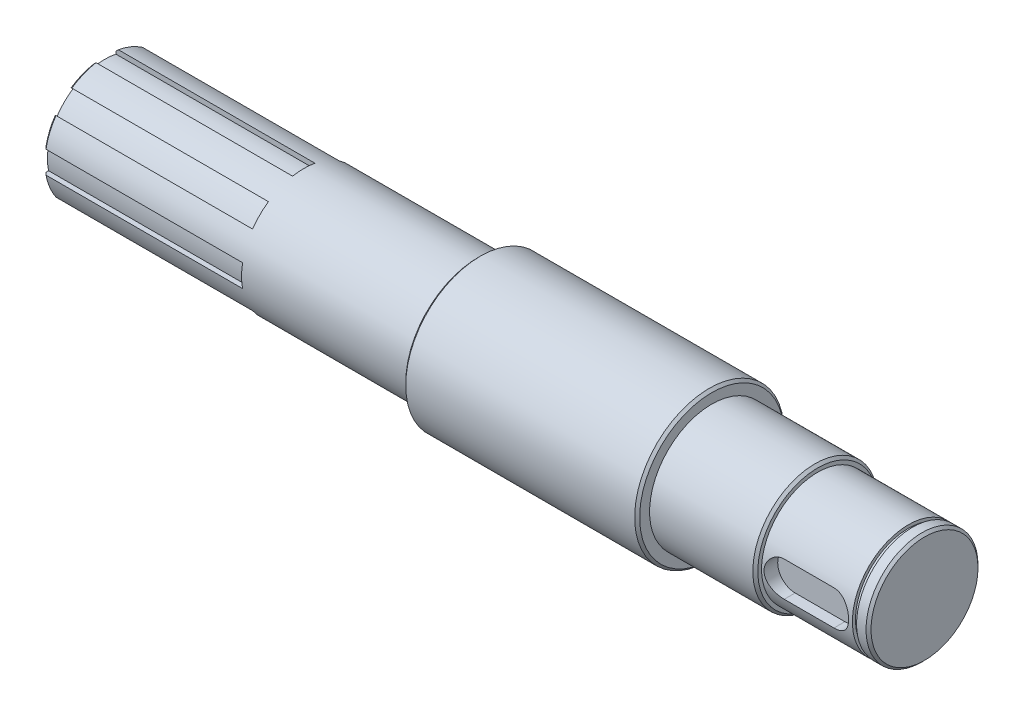
from build123d import *

# Parameters (mm, degrees)
CHAMFER_1_SIZE      = 1
CUT_EXTRUDE_START   = 1.7
SKETCH_2_R          = 22.5
SKETCH_2_R_2        = 21.25
CUT_EXTRUDE_1_DEPTH = 1.7
CUT_EXTRUDE_2_DEPTH = 5.5
CUT_EXTRUDE_START_2 = -80
CUT_EXTRUDE_3_DEPTH = 80
CHAMFER_2_SIZE      = 1


with BuildPart() as part:
    # 草图1 → 旋转1 (revolve)
    with BuildSketch(Plane.XY, mode=Mode.PRIVATE) as revolve_1_sk:
        Polygon((0, 0), (0, 25), (150, 25), (150, 30), (244, 30), (244, 25), (286.5, 25), (286.5, 22.5), (329.5, 22.5), (329.5, 0), align=None)
    revolve(revolve_1_sk.sketch.rotate(Axis((329.5, 0, 0), (-1, 0, 0)), 90), axis=Axis((329.5, 0, 0), (-1, 0, 0)))

    # 倒角1
    chamfer_1_edges = [part.edges().sort_by_distance(p)[0] for p in [
        (329.5, 0, 22.5),
        (286.5, 0, 25),
        (244, 0, 30),
        (150, 0, 30),
    ]]
    chamfer(chamfer_1_edges, length=CHAMFER_1_SIZE)

    # 草图2 → 切除-拉伸1 (cut)
    with BuildSketch(Plane(origin=(323, 0, 0), x_dir=(0, 0, -1), z_dir=(1, 0, 0)).offset(CUT_EXTRUDE_START)):
        Circle(SKETCH_2_R)
        Circle(SKETCH_2_R_2, mode=Mode.SUBTRACT)
    extrude(amount=-CUT_EXTRUDE_1_DEPTH, mode=Mode.SUBTRACT)

    # 草图3 → 切除-拉伸2 (cut)
    with BuildSketch(Plane.XY.offset(22.5)):
        with BuildLine():
            Line((294.5, 7), (314.5, 7))
            ThreePointArc((314.5, 7), (321.5, 0), (314.5, -7))
            Line((314.5, -7), (294.5, -7))
            ThreePointArc((294.5, -7), (287.5, 0), (294.5, 7))
        make_face()
    extrude(amount=-CUT_EXTRUDE_2_DEPTH, mode=Mode.SUBTRACT)

    # 草图4 → 切除-拉伸3 (cut)
    with BuildSketch(Plane.ZY.offset(CUT_EXTRUDE_START_2)):
        with BuildLine():
            Line((-4.5, 24.591665255), (-4.5, 22.555487137))
            ThreePointArc((-4.5, 22.555487137), (0, 23), (4.5, 22.555487137))
            Line((4.5, 22.555487137), (4.5, 24.591665255))
            ThreePointArc((4.5, 24.591665255), (0, 25), (-4.5, 24.591665255))
        make_face()
        with BuildLine():
            Line((20.570913778, 14.206952747), (19.131118423, 12.767157392))
            ThreePointArc((19.131118423, 12.767157392), (16.263455967, 16.263455967), (12.767157392, 19.131118423))
            Line((12.767157392, 19.131118423), (14.206952747, 20.570913778))
            ThreePointArc((14.206952747, 20.570913778), (17.67766953, 17.67766953), (20.570913778, 14.206952747))
        make_face()
        with BuildLine():
            Line((24.591665255, -4.5), (22.555487137, -4.5))
            ThreePointArc((22.555487137, -4.5), (23, 0), (22.555487137, 4.5))
            Line((22.555487137, 4.5), (24.591665255, 4.5))
            ThreePointArc((24.591665255, 4.5), (25, 0), (24.591665255, -4.5))
        make_face()
        with BuildLine():
            Line((14.206952747, -20.570913778), (12.767157392, -19.131118423))
            ThreePointArc((12.767157392, -19.131118423), (16.263455967, -16.263455967), (19.131118423, -12.767157392))
            Line((19.131118423, -12.767157392), (20.570913778, -14.206952747))
            ThreePointArc((20.570913778, -14.206952747), (17.67766953, -17.67766953), (14.206952747, -20.570913778))
        make_face()
        with BuildLine():
            Line((-4.5, -24.591665255), (-4.5, -22.555487137))
            ThreePointArc((-4.5, -22.555487137), (0, -23), (4.5, -22.555487137))
            Line((4.5, -22.555487137), (4.5, -24.591665255))
            ThreePointArc((4.5, -24.591665255), (0, -25), (-4.5, -24.591665255))
        make_face()
        with BuildLine():
            Line((-20.570913778, -14.206952747), (-19.131118423, -12.767157392))
            ThreePointArc((-19.131118423, -12.767157392), (-16.263455967, -16.263455967), (-12.767157392, -19.131118423))
            Line((-12.767157392, -19.131118423), (-14.206952747, -20.570913778))
            ThreePointArc((-14.206952747, -20.570913778), (-17.67766953, -17.67766953), (-20.570913778, -14.206952747))
        make_face()
        with BuildLine():
            Line((-24.591665255, 4.5), (-22.555487137, 4.5))
            ThreePointArc((-22.555487137, 4.5), (-23, 0), (-22.555487137, -4.5))
            Line((-22.555487137, -4.5), (-24.591665255, -4.5))
            ThreePointArc((-24.591665255, -4.5), (-25, 0), (-24.591665255, 4.5))
        make_face()
        with BuildLine():
            Line((-14.206952747, 20.570913778), (-12.767157392, 19.131118423))
            ThreePointArc((-12.767157392, 19.131118423), (-16.263455967, 16.263455967), (-19.131118423, 12.767157392))
            Line((-19.131118423, 12.767157392), (-20.570913778, 14.206952747))
            ThreePointArc((-20.570913778, 14.206952747), (-17.67766953, 17.67766953), (-14.206952747, 20.570913778))
        make_face()
    extrude(amount=CUT_EXTRUDE_3_DEPTH, mode=Mode.SUBTRACT)

    # 倒角2
    chamfer_2_edges = [part.edges().sort_by_distance(p)[0] for p in [
        (0, 23.096988313, 9.567085809),
        (0, 9.567085809, 23.096988313),
        (0, -9.567085809, 23.096988313),
        (0, -23.096988313, 9.567085809),
        (0, -23.096988313, -9.567085809),
        (0, -9.567085809, -23.096988313),
        (0, 9.567085809, -23.096988313),
        (0, 23.096988313, -9.567085809),
    ]]
    chamfer(chamfer_2_edges, length=CHAMFER_2_SIZE)


solid = part.part
